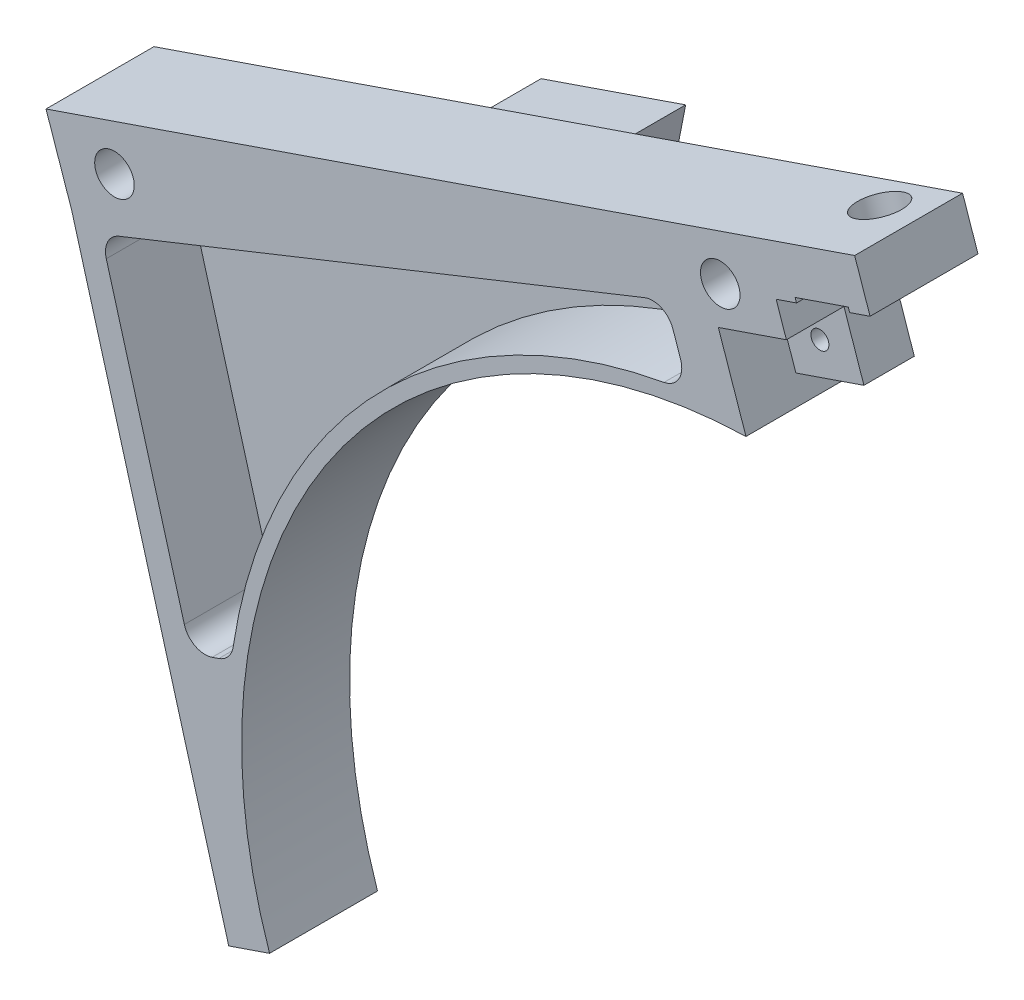
SolidWorks part; units mm, degrees
ref_plane "前视基准面" through (0, 0, 0) normal (0, 0, 1) x (1, 0, 0)
ref_plane "上视基准面" through (0, 0, 0) normal (0, 1, 0) x (1, 0, 0)
ref_plane "右视基准面" through (0, 0, 0) normal (1, 0, 0) x (0, 0, -1)
sketch "草图1" plane through (0, 0, 0) normal (0, 0, 1) x (1, 0, 0)
  line L12 (154.5015, 74.3658) -> (160.1778, 76.31)
  line L13 (230.5708, 190.2259) -> (233.4085, 191.1994)
  line L26 (132.6806, 151.9915) -> (154.5015, 74.3658)
  line L31 (129.1111, 162.3962) -> (132.6806, 151.9915)
  line L32 (129.1111, 162.3962) -> (241.4823, 200.9469)
  line L33 (241.4823, 200.9469) -> (243.624, 194.704)
  line L34 (243.624, 194.704) -> (240.7864, 193.7305)
  line L35 (240.7864, 193.7305) -> (240.5917, 194.298)
  line L36 (240.5917, 194.298) -> (233.2138, 191.7669)
  line L37 (233.2138, 191.7669) -> (233.4085, 191.1994)
  line L38 (231.9986, 186.064) -> (230.5708, 190.2259)
  line L39 (234.7722, 177.9663) -> (231.9986, 186.064)
  line L40 (234.7722, 177.9663) -> (225.3157, 174.7273)
  line L41 (226.3833, 171.6154) -> (225.3157, 174.7273)
  arc A0 (160.1778, 76.31) -> (270.9125, 41.6099) centre (228.293, 99.6407) ccw construction
  arc A1 (226.3833, 171.6154) -> (160.1778, 76.31) centre (228.293, 99.6407) ccw
extrude "凸台-拉伸1" add sketch "草图1" along normal blind 15 contours L26 L12 A1 L41 L40 L39 L38 L13 L37 L36 L35 L34 L33 L32 L31
sketch "草图2" plane through (0, 0, 0) normal (0, 0, -1) x (-1, 0, 0)
  line L0 (-175.3819, 177.6036) -> (-194.5243, 184.1707) construction
  line L1 (-181.1198, 172.03) -> (-175.2859, 177.1129) construction
  line L2 (-194.9013, 183.8423) -> (-193.4163, 176.2485) construction
  line L3 (-193.6974, 175.4293) -> (-234.9219, 189.572) construction
  line L4 (-174.9089, 177.4414) -> (-194.9973, 184.333)
  line L5 (-181.8738, 171.3731) -> (-174.9089, 177.4414)
  line L6 (-194.9973, 184.333) -> (-193.2244, 175.2671)
  line L7 (-181.8738, 171.3731) -> (-193.2244, 175.2671)
extrude "凸台-拉伸2" add sketch "草图2" along normal up to surface (8 mm away)
sketch "草图3" plane through (0, 0, 15) normal (0, 0, 1) x (1, 0, 0)
  line L8 (154.5015, 74.3658) -> (160.1778, 76.31) construction
  line L9 (148.3358, 109.9739) -> (137.489, 148.5606)
  line L10 (153.1245, 108.2662) -> (152.1974, 107.9481)
  line L11 (217.2976, 176.3615) -> (216.2336, 179.4628)
  line L12 (212.2848, 181.2759) -> (139.2658, 152.159)
  arc A0 (265.6976, 25.3341) -> (267.7055, 29.1876) centre (264.8669, 28.2169) ccw construction
  arc A1 (266.6446, 32.2899) -> (262.4224, 33.9811) centre (263.806, 31.3192) ccw construction
  arc A3 (177.2387, 46.0733) -> (174.1982, 46.7403) centre (175.1689, 43.9017) ccw construction
  arc A4 (173.2708, 46.4231) -> (171.4622, 42.4552) centre (174.2415, 43.5845) ccw construction
  arc A5 (186.5509, 5.3214) -> (190.1609, 3.5681) centre (189.3302, 6.4508) ccw construction
  arc A12 (137.489, 148.5606) -> (139.2658, 152.159) centre (140.377, 149.3724) cw
  arc A13 (152.1974, 107.9481) -> (148.3358, 109.9739) centre (151.2239, 110.7858) cw
  arc A14 (155.1176, 110.6572) -> (153.1245, 108.2662) centre (152.151, 111.1038) cw
  arc A15 (155.1176, 110.6572) -> (214.9989, 172.4368) centre (228.293, 99.6407) cw
  arc A16 (217.2976, 176.3615) -> (214.9989, 172.4368) centre (214.4599, 175.388) cw
  arc A17 (212.2848, 181.2759) -> (216.2336, 179.4628) centre (213.396, 178.4893) cw
extrude "切除-拉伸1" cut sketch "草图3" against normal blind 12
sketch "草图4" plane through (0, 0, 15) normal (0, 0, 1) x (1, 0, 0)
  line L1 (274.7451, 30.4025) -> (284.2071, 33.6382) construction
  line L3 (281.4335, 41.7359) -> (271.977, 38.4969) construction
  line L8 (154.5015, 74.3658) -> (160.1778, 76.31) construction
  line L9 (234.7722, 177.9663) -> (225.3157, 174.7273)
  line L10 (234.7722, 177.9663) -> (231.9986, 186.064)
  line L11 (222.5397, 182.819) -> (231.9986, 186.064)
  line L12 (225.3157, 174.7273) -> (222.5397, 182.819)
extrude "切除-拉伸2" cut sketch "草图4" against normal blind 8
sketch "草图5" plane through (0, 0, 15) normal (0, 0, 1) x (1, 0, 0)
  line L0 (154.5015, 74.3658) -> (160.1778, 76.31) construction
  circle A0 centre (278.0907, 36.0684) radius 1.5 construction
  circle A2 centre (228.6566, 180.3942) radius 0.5
  dimension "D1" = 1
extrude "切除-拉伸3" cut sketch "草图5" against normal through all
sketch "草图6" plane through (0, 0, 15) normal (0, 0, 1) x (1, 0, 0)
  line L0 (154.5015, 74.3658) -> (160.1778, 76.31) construction
  circle A0 centre (278.2554, 26.3186) radius 2.75 construction
  circle A1 centre (194.0433, -2.4794) radius 2.75 construction
  circle A4 centre (138.6252, 159.3169) radius 2.75
  circle A5 centre (222.809, 188.1974) radius 2.75
extrude "切除-拉伸4" cut sketch "草图6" against normal through all
hole_wizard "Ø3.0 (3) 直径孔1" positions "草图7" profile "草图8" hole size "Ø3.0" standard "GB" end condition through all
sketch "草图7" plane through (-34.3035, 99.9912, 0) normal (0.3245, -0.9459, 0) x (-0.9459, -0.3245, 0)
  point P0 (-286.7219, -5)
sketch "草图8" plane through (236.9027, 193.0325, 5) normal (0, 0, 1) x (0.9459, 0.3245, 0)
  line L0 (0, 0) -> (0, 42.4645)
  line L1 (0, 42.4645) -> (3.25, 42.4645)
  line L2 (3.25, 42.4645) -> (3.25, 0)
  line L5 (3.25, 0) -> (0, 0)
  line L11 (0, -6.35) -> (0, 107.95) construction
  dimension "通孔孔直径" = 6.5
  dimension "通孔孔深度" = 42.4645
hole_wizard "M3 螺纹孔1" positions "草图9" profile "草图10" tap size "M3" standard "GB" end condition through all
sketch "草图9" plane through (0, 0, 7) normal (0, 0, 1) x (1, 0, 0)
  point P0 (228.6566, 180.3942)
sketch "草图10" plane through (228.6566, 180.3942, 7) normal (1, 0, 0) x (0, -1, 0)
  line L0 (0, 0) -> (0, 15)
  line L1 (0, 15) -> (1.25, 15)
  line L2 (1.25, 15) -> (1.25, 0)
  line L5 (1.25, 0) -> (0, 0)
  line L11 (0, -6.35) -> (0, 107.95) construction
  dimension "通孔螺纹孔钻头直径" = 2.5
  dimension "通孔螺纹孔钻头深度" = 15
cosmetic thread "孔螺蚊线1" parameters "D2"=3
